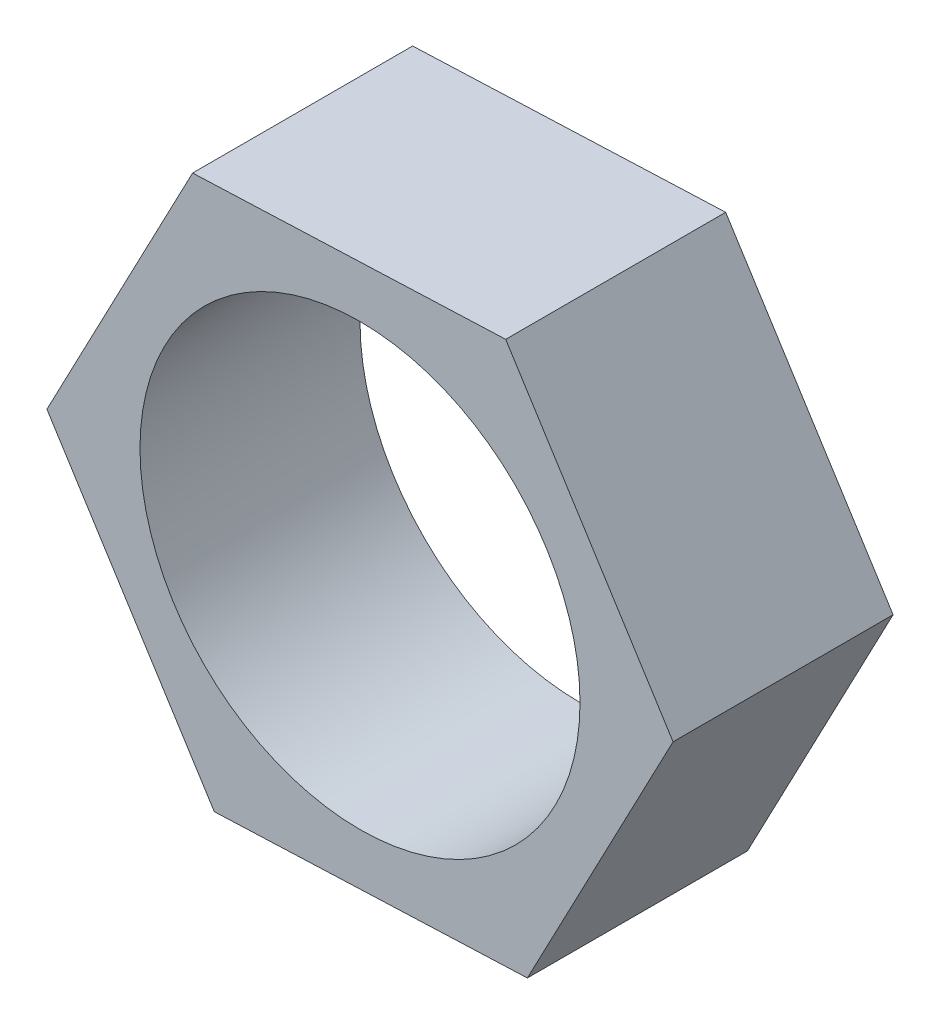
SolidWorks part; units mm, degrees
ref_plane "Front Plane" through (0, 0, 0) normal (0, 0, 1) x (1, 0, 0)
ref_plane "Top Plane" through (0, 0, 0) normal (0, 1, 0) x (1, 0, 0)
ref_plane "Right Plane" through (0, 0, 0) normal (1, 0, 0) x (0, 0, -1)
other "Configuration Table"
sketch "Sketch1" plane through (0, 0, 0) normal (0, 0, 1) x (1, 0, 0)
  line L1 (9.9327, 18.9123) -> (-11.4122, 18.0581)
  line L2 (-11.4122, 18.0581) -> (-21.3449, -0.8542)
  line L3 (-21.3449, -0.8542) -> (-9.9327, -18.9123)
  line L4 (-9.9327, -18.9123) -> (11.4122, -18.0581)
  line L5 (11.4122, -18.0581) -> (21.3449, 0.8542)
  line L6 (21.3449, 0.8542) -> (9.9327, 18.9123)
  circle A0 centre (0, 0) radius 18.5 construction
  circle A1 centre (0, 0) radius 15
  dimension "D1" = 37
  dimension "D2" = 30
extrude "Boss-Extrude1" add sketch "Sketch1" along normal blind 15
